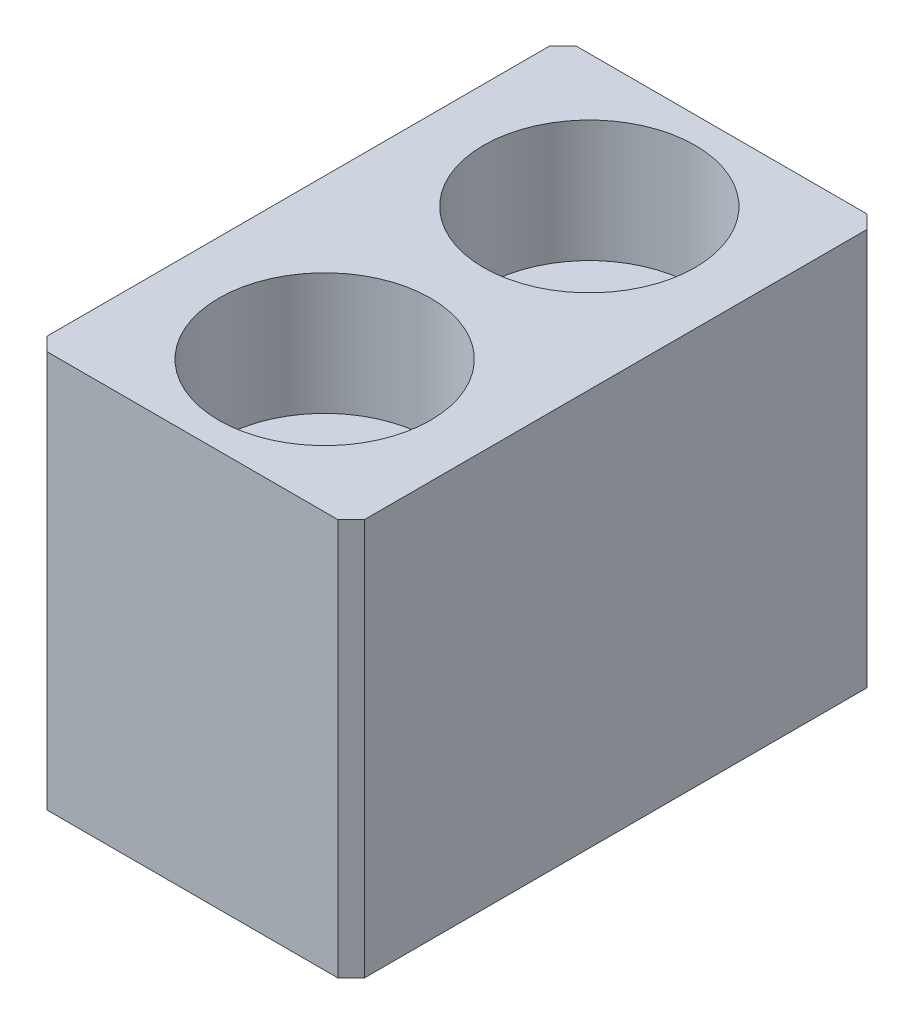
SolidWorks part; units mm, degrees
material "优力胶"
ref_plane "前视基准面" through (0, 0, 0) normal (0, 0, 1) x (1, 0, 0)
ref_plane "上视基准面" through (0, 0, 0) normal (0, 1, 0) x (1, 0, 0)
ref_plane "右视基准面" through (0, 0, 0) normal (1, 0, 0) x (0, 0, -1)
sketch "草图1" plane through (0, 0, 0) normal (0, 1, 0) x (1, 0, 0)
  line L1 (-6, 10) -> (6, 10)
  line L2 (-6, 10) -> (-6, -10)
  line L3 (-6, -10) -> (6, -10)
  line L4 (6, 10) -> (6, -10)
  line L5 (-6, 10) -> (6, -10) construction
  line L6 (-6, -10) -> (6, 10) construction
  point P0 (0, 0)
  dimension "D1" = 12
  dimension "D2" = 20
extrude "凸台-拉伸1" add sketch "草图1" along normal blind 15
hole_wizard "打孔尺寸(%根据)内六角圆柱头螺钉的类型1" positions "草图2" profile "草图3" counterbore size "M4" standard "GB"
sketch "草图2" plane through (0, 15, 0) normal (0, 1, 0) x (1, 0, 0)
  line L0 (6, 10) -> (-6, 10) construction
  line L1 (-6, -10) -> (6, -10) construction
  line L2 (-6, 10) -> (-6, -10) construction
  point P0 (0, 5)
  point P2 (0, -5)
  dimension "D1" = 5
  dimension "D2" = 5
  dimension "D3" = 6
sketch "草图3" plane through (0, 15, -5) normal (1, 0, 0) x (0, 0, 1)
  line L0 (0, 0) -> (0, 21.3519)
  line L1 (0, 21.3519) -> (2.25, 20)
  line L2 (2.25, 20) -> (2.25, 4.6)
  line L3 (2.25, 4.6) -> (4, 4.6)
  line L4 (4, 4.6) -> (4, 0)
  line L5 (4, 0) -> (0, 0)
  line L10 (0, 21.3519) -> (-2.25, 20) construction
  line L11 (0, -6.35) -> (0, 107.95) construction
  dimension "孔直径" = 4.5
  dimension "孔深度" = 20
  dimension "柱形沉头孔直径" = 8
  dimension "柱形沉头孔深度" = 4.6
  dimension "导头角度" = 118
chamfer "倒角1" distance 0.5 angle 45 4 edges at (6, 7.5, -10) (6, 7.5, 10) (-6, 7.5, 10) (-6, 7.5, -10)
